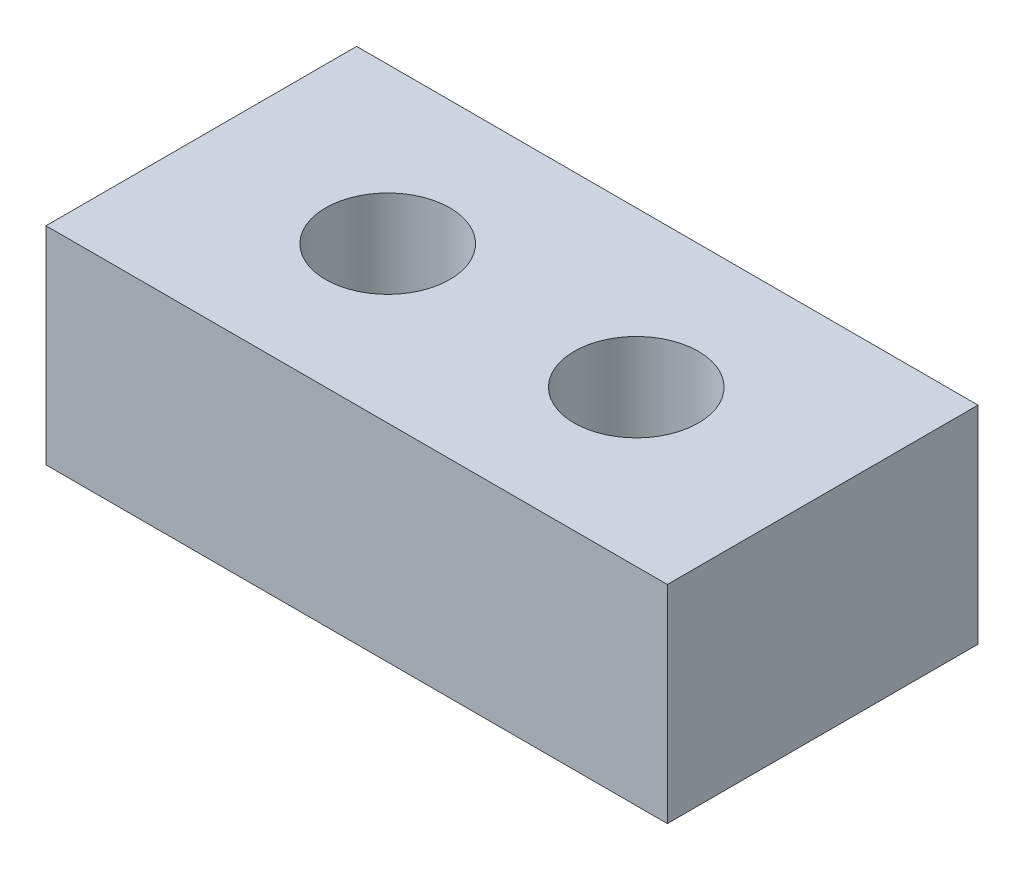
from build123d import *

# Parameters (mm, degrees)
SKETCH1_W           = 300
SKETCH1_H           = 150
SKETCH1_R           = 30
BOSS_EXTRUDE1_DEPTH = 50


with BuildPart() as part:
    # Sketch1 → Boss-Extrude1 (new, symmetric)
    with BuildSketch(Plane(origin=(0, 0, 0), x_dir=(1, 0, 0), z_dir=(0, 1, 0))):
        Rectangle(SKETCH1_W, SKETCH1_H)
        with Locations(Location((60, 0, 0), (0, 0, 90))):
            Circle(SKETCH1_R, mode=Mode.SUBTRACT)
        with Locations(Location((-60, 0, 0), (0, 0, 90))):
            Circle(SKETCH1_R, mode=Mode.SUBTRACT)
    extrude(amount=BOSS_EXTRUDE1_DEPTH, both=True)


solid = part.part
